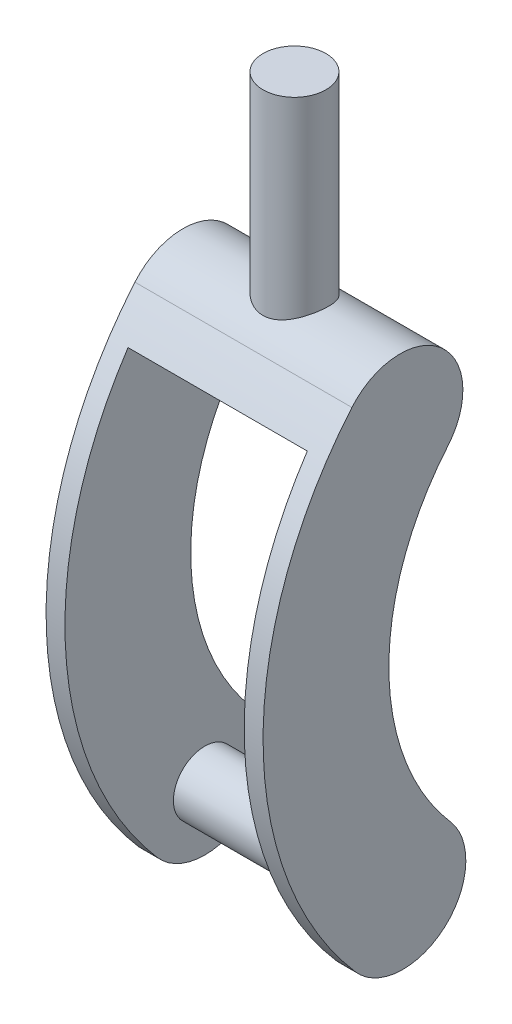
from build123d import *

# Parameters (mm, degrees)
BOSS_EXTRUDE1_DEPTH             = 34.5
SKETCH2_R                       = 100
CUT_EXTRUDE1_DEPTH              = 28.5
CUT_EXTRUDE2_DEPTH              = 57
SKETCH5_R                       = 10
BOSS_EXTRUDE2_DEPTH             = 29
BOSS_EXTRUDE3_REACH             = 229.088
BOSS_EXTRUDE3_END_RADIUS        = 20
SKETCH7_R                       = 10
BOSS_EXTRUDE3_DIRECTION_2_DEPTH = 10


with BuildPart() as part:
    # Sketch1 → Boss-Extrude1 (new, symmetric)
    with BuildSketch(Plane(origin=(0, 0, 0), x_dir=(0, 0, -1), z_dir=(1, 0, 0))):
        with BuildLine():
            ThreePointArc((-16.232839847, 142.89001702), (-44.477266745, 64.681536406), (-15.103918242, -13.10998298))
            ThreePointArc((-15.103918242, -13.10998298), (13.10998298, -15.103918242), (15.103918242, 13.10998298))
            ThreePointArc((15.103918242, 13.10998298), (-4.478314094, 64.970995905), (14.351303838, 117.10998298))
            ThreePointArc((14.351303838, 117.10998298), (11.949249015, 145.292071843), (-16.232839847, 142.89001702))
        make_face()
    extrude(amount=BOSS_EXTRUDE1_DEPTH, both=True)

    # Sketch2 → Cut-Extrude1 (cut, symmetric)
    with BuildSketch(Plane(origin=(0, 0, 0), x_dir=(0, 0, -1), z_dir=(1, 0, 0))):
        Circle(SKETCH2_R)
    extrude(amount=CUT_EXTRUDE1_DEPTH, both=True, mode=Mode.SUBTRACT)

    # Sketch4 → Cut-Extrude2 (cut)
    with BuildSketch(Plane.ZY.offset(-28.5)):
        Polygon((-31.404068156, 111.748185713), (46.911557074, 140.123412246), (75.162269232, 67.90846072), (-19.75286352, 46.910793085), align=None)
    extrude(amount=CUT_EXTRUDE2_DEPTH, mode=Mode.SUBTRACT)

    # Sketch5 → Boss-Extrude2 (add, symmetric)
    with BuildSketch(Plane(origin=(0, 0, 0), x_dir=(0, 0, -1), z_dir=(1, 0, 0))):
        Circle(SKETCH5_R)
    extrude(amount=BOSS_EXTRUDE2_DEPTH, both=True)

    # Boss-Extrude3: up to this cylinder (the profile starts outside it)
    boss_extrude3_end = Plane(origin=(0, 130, 0.940768004), z_dir=(-1, 0, 0)) * Cylinder(BOSS_EXTRUDE3_END_RADIUS, 499.176, mode=Mode.PRIVATE)
    # Sketch7 → Boss-Extrude3 (add, up to the surface)
    with BuildSketch(Plane(origin=(0, 200, 0), x_dir=(1, 0, 0), z_dir=(0, 1, 0)), mode=Mode.PRIVATE) as boss_extrude3_sk1:
        with Locations(Location((0, 0, 0), (0, 0, 90))):
            Circle(SKETCH7_R)
    boss_extrude3_tool1 = extrude(boss_extrude3_sk1.sketch, amount=-BOSS_EXTRUDE3_REACH, mode=Mode.PRIVATE) - boss_extrude3_end
    add(boss_extrude3_tool1.solids().sort_by_distance((0, 200, 0))[0])

    # Sketch7 → Boss-Extrude3 direction 2 (add)
    with BuildSketch(Plane(origin=(0, 200, 0), x_dir=(1, 0, 0), z_dir=(0, 1, 0))):
        with Locations(Location((0, 0, 0), (0, 0, 90))):
            Circle(SKETCH7_R)
    extrude(amount=BOSS_EXTRUDE3_DIRECTION_2_DEPTH)


solid = part.part
